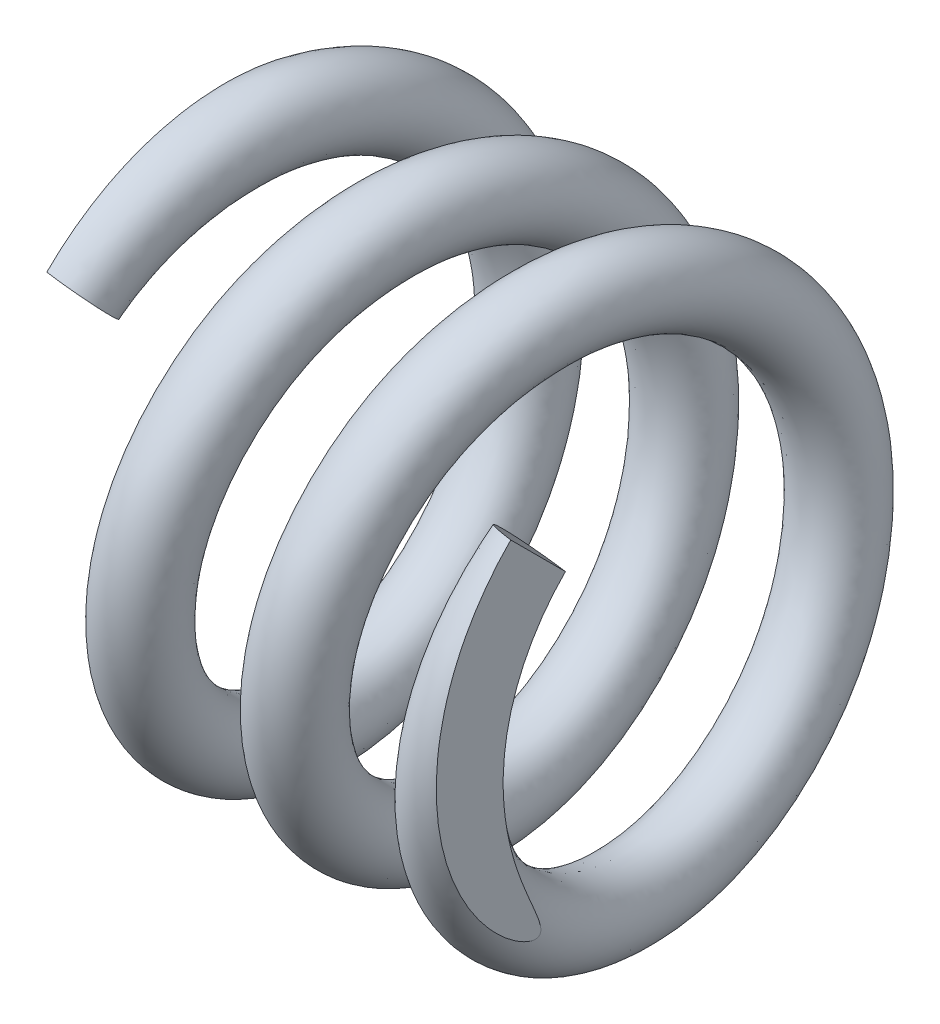
from build123d import *

# Parameters (mm, degrees)
SWEEP1_PITCH            = 1
SWEEP1_HEIGHT           = 3
SWEEP1_RADIUS           = 1.5
SWEEP1_START_ANGLE      = -45
SWEEP1_PROFILE_R        = 0.25
CUT_EXTRUDE2_DEPTH      = 5.083922994
CUT_EXTRUDE2_DEPTH_BACK = 5.083922994
SKETCH8_OUTSIDE_W       = 6.71
SKETCH8_OUTSIDE_H       = 6.712
SKETCH8_OUTSIDE_W_2     = 3
SKETCH8_OUTSIDE_H_2     = 5.007784657


with BuildPart() as part:
    # Sweep1: sweep along a helix
    with BuildLine() as sweep1_path:
        add(Helix(SWEEP1_PITCH, SWEEP1_HEIGHT, SWEEP1_RADIUS, center=(0, 0, 0), direction=(1, 0, 0), lefthand=True, mode=Mode.PRIVATE).rotate(Axis((0, 0, 0), (1, 0, 0)), SWEEP1_START_ANGLE))
    # Sweep1 profile (on start of the path) → Sweep1 (sweep)
    with BuildSketch(Plane(origin=(0, 1.060660172, 1.060660172), x_dir=(0, 0.7071067811865146, 0.7071067811865807), z_dir=(0.1055110407535529, 0.7031598041267698, -0.7031598041267042))):
        Circle(SWEEP1_PROFILE_R)
    sweep(path=sweep1_path.line, is_frenet=True)

    # Sketch8 outside → Cut-Extrude2 (cut, two sides: drawn at the far end of the back side and taken through both)
    with BuildSketch(Plane.XY.offset(-CUT_EXTRUDE2_DEPTH_BACK)):
        with Locations((1.5, 0)):
            Rectangle(SKETCH8_OUTSIDE_W, SKETCH8_OUTSIDE_H)
        with Locations((1.5, -0.22356974)):
            Rectangle(SKETCH8_OUTSIDE_W_2, SKETCH8_OUTSIDE_H_2, mode=Mode.SUBTRACT)
    extrude(amount=CUT_EXTRUDE2_DEPTH + CUT_EXTRUDE2_DEPTH_BACK, mode=Mode.SUBTRACT)


solid = part.part
